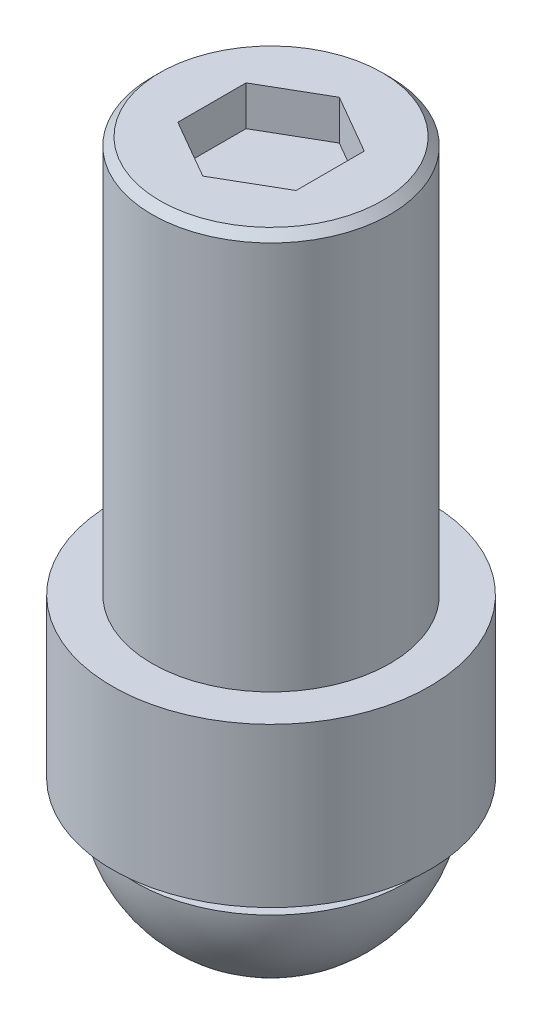
SolidWorks part; units mm, degrees
material "Q235A"
ref_plane "Front Plane" through (0, 0, 0) normal (0, 0, 1) x (1, 0, 0)
ref_plane "Top Plane" through (0, 0, 0) normal (0, 1, 0) x (1, 0, 0)
ref_plane "Right Plane" through (0, 0, 0) normal (1, 0, 0) x (0, 0, -1)
sketch "Sketch1" plane through (0, 0, 0) normal (0, 1, 0) x (1, 0, 0)
  circle A0 centre (0, 0) radius 1.5
  dimension "D1" = 3
extrude "Boss-Extrude1" add sketch "Sketch1" along normal blind 5
sketch "Sketch2" plane through (0, 0, 0) normal (0, -1, 0) x (1, 0, 0)
  circle A0 centre (0, 0) radius 2
  dimension "D1" = 4
extrude "Boss-Extrude2" add sketch "Sketch2" along normal blind 2
sketch "Sketch3" plane through (0, 0, 0) normal (0, 0, 1) x (1, 0, 0)
  line L0 (0, -2) -> (0, -3.7987)
  line L1 (-2, -2) -> (2, -2) construction
  line L2 (0, -2) -> (1.3767, -2)
  line L3 (1.3767, -2) -> (1.3767, -2.2944)
  line L4 (1.3767, -2.2944) -> (1.7, -2.2944)
  arc A0 (0, -3.7987) -> (1.7, -2.2944) centre (0, -2.086) ccw
  dimension "1.7" = 1.7
revolve "Revolve1" add sketch "Sketch3" angle 360 about L0
sketch "Sketch4" plane through (0, 5, 0) normal (0, 1, 0) x (1, 0, 0)
  line L1 (0, 0.8602) -> (-0.7449, 0.4301)
  line L2 (-0.7449, 0.4301) -> (-0.7449, -0.4301)
  line L3 (-0.7449, -0.4301) -> (0, -0.8602)
  line L4 (0, -0.8602) -> (0.7449, -0.4301)
  line L5 (0.7449, -0.4301) -> (0.7449, 0.4301)
  line L6 (0.7449, 0.4301) -> (0, 0.8602)
  circle A0 centre (0, 0) radius 0.7449 construction
extrude "Cut-Extrude1" cut sketch "Sketch4" against normal blind 0.5
chamfer "Chamfer1" distance 0.1 angle 45 1 edges at (0, 5, 1.5)
